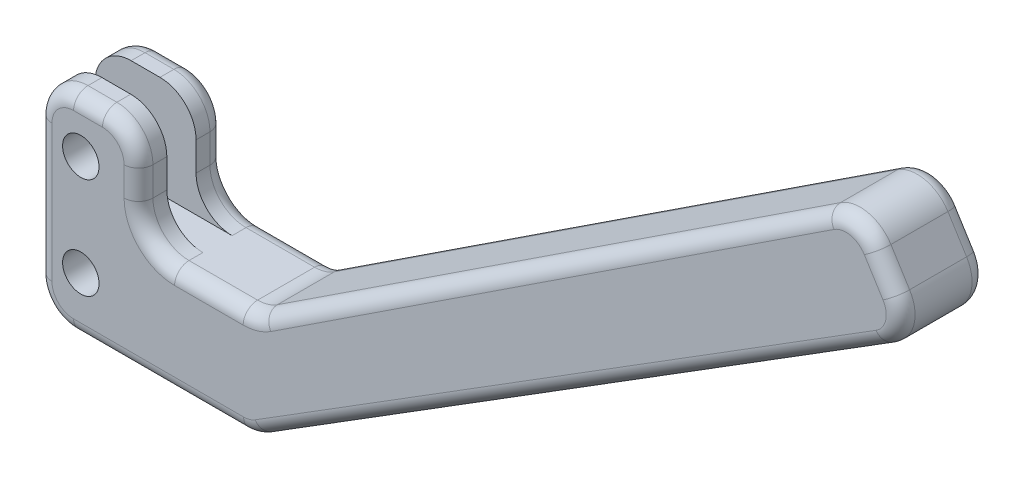
from build123d import *

# Parameters (mm, degrees)
SKETCH1_W           = 30
SKETCH1_H           = 15
BOSS_EXTRUDE1_DEPTH = 11.9
SKETCH2_W           = 14
SKETCH2_H           = 14
BOSS_EXTRUDE2_DEPTH = 11.9
SKETCH3_R           = 2.525
SKETCH3_R_2         = 1.65
CUT_EXTRUDE2_DEPTH  = 11.9
BOSS_EXTRUDE3_DEPTH = 11.9
SKETCH5_W           = 14
SKETCH5_H           = 4.05
CUT_EXTRUDE3_DEPTH  = 26
FILLET1_R           = 5
FILLET2_R           = 2
SKETCH6_R           = 2.525
CUT_EXTRUDE4_DEPTH  = 3.925


with BuildPart() as part:
    # Sketch1 → Boss-Extrude1 (new body)
    with BuildSketch(Plane.XY):
        Rectangle(SKETCH1_W, SKETCH1_H)
    extrude(amount=BOSS_EXTRUDE1_DEPTH)

    # Sketch2 → Boss-Extrude2 (add)
    with BuildSketch(Plane.XY.offset(11.9)):
        with Locations((-8, 14.5)):
            Rectangle(SKETCH2_W, SKETCH2_H)
    extrude(amount=-BOSS_EXTRUDE2_DEPTH)

    # Sketch3 → Cut-Extrude2 (cut)
    with BuildSketch(Plane.XY.offset(11.9)):
        with Locations((-9, 0.5)):
            Circle(SKETCH3_R)
        with Locations((-9, 14.5)):
            Circle(SKETCH3_R_2)
    extrude(amount=-CUT_EXTRUDE2_DEPTH, mode=Mode.SUBTRACT)

    # Sketch4 → Boss-Extrude3 (add)
    with BuildSketch(Plane.XY.offset(11.9)):
        Polygon((15, -7.5), (106.523733582, 49.690376088), (98.574944619, 62.41109753), (15, 7.5), align=None)
    extrude(amount=-BOSS_EXTRUDE3_DEPTH)

    # Sketch5 → Cut-Extrude3 (cut)
    with BuildSketch(Plane(origin=(0, 7.5, 0), x_dir=(1, 0, 0), z_dir=(0, 1, 0))):
        with Locations((-8, -5.95)):
            Rectangle(SKETCH5_W, SKETCH5_H)
    extrude(amount=CUT_EXTRUDE3_DEPTH, mode=Mode.SUBTRACT)

    # Fillet1
    fillet1_edges = [part.edges().sort_by_distance(p)[0] for p in [
        (-15, 21.5, 1.9625),
        (-1, 21.5, 1.9625),
        (-1, 7.5, 1.9625),
        (98.574944619, 62.41109753, 5.95),
        (106.523733582, 49.690376088, 5.95),
        (-1, 21.5, 9.9375),
        (-1, 7.5, 9.9375),
        (-15, 21.5, 9.9375),
        (15, -7.5, 5.95),
        (-15, -7.5, 5.95),
        (15, 7.5, 5.95),
    ]]
    fillet(fillet1_edges, radius=FILLET1_R)

    # Fillet2
    fillet2_edges = [part.edges().sort_by_distance(p)[0] for p in [
        (14.937271043, 7.709711065, 0),
        (14.937271043, 7.709711065, 11.9),
        (0.464466094, 8.964466094, 11.9),
        (0.464466094, 8.964466094, 0),
        (102.579887045, 56.001849878, 0),
        (102.579887045, 56.001849878, 11.9),
        (1.783136536, -7.5, 11.9),
        (59.249681247, 20.150269643, 11.9),
        (55.274895994, 33.961743433, 11.9),
        (8.75219782, 7.5, 11.9),
        (-1, 14.5, 11.9),
        (-8, 21.5, 11.9),
        (-15, 7, 11.9),
        (-13.535533906, 20.035533906, 11.9),
        (-2.464466094, 20.035533906, 11.9),
        (-13.535533906, -6.035533906, 11.9),
        (14.94445985, -7.30630848, 11.9),
        (104.505747104, 50.156264976, 11.9),
        (98.114553442, 60.307839752, 11.9),
        (55.274895994, 33.961743433, 0),
        (8.75219782, 7.5, 0),
        (59.249681247, 20.150269643, 0),
        (1.783136536, -7.5, 0),
        (-15, 7, 0),
        (-8, 21.5, 0),
        (-1, 14.5, 0),
        (-13.535533906, 20.035533906, 0),
        (-2.464466094, 20.035533906, 0),
        (-13.535533906, -6.035533906, 0),
        (14.94445985, -7.30630848, 0),
        (104.505747104, 50.156264976, 0),
        (98.114553442, 60.307839752, 0),
    ]]
    fillet(fillet2_edges, radius=FILLET2_R)

    # Sketch6 → Cut-Extrude4 (cut)
    with BuildSketch(Plane.XY.offset(11.9)):
        with Locations((-9, 14.5)):
            Circle(SKETCH6_R)
    extrude(amount=-CUT_EXTRUDE4_DEPTH, mode=Mode.SUBTRACT)


solid = part.part
